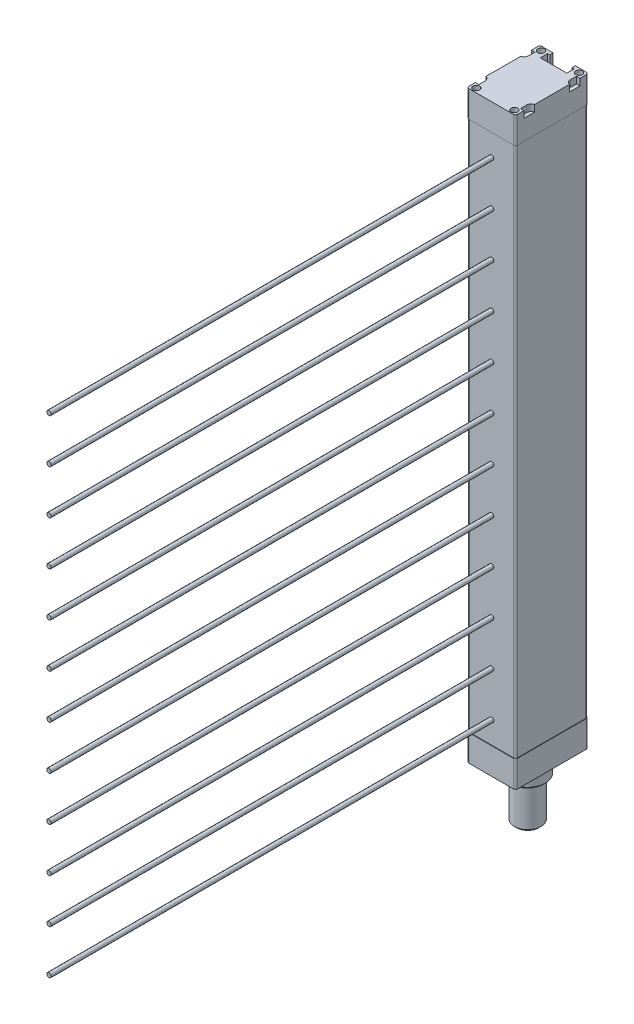
SolidWorks part; units mm, degrees
material "A6061"
ref_plane "前基準面" through (0, 0, 0) normal (0, 0, 1) x (1, 0, 0)
ref_plane "上基準面" through (0, 0, 0) normal (0, 1, 0) x (1, 0, 0)
ref_plane "右基準面" through (0, 0, 0) normal (1, 0, 0) x (0, 0, -1)
sketch "草圖1" plane through (0, 0, 0) normal (0, 1, 0) x (1, 0, 0)
  line L0 (-11, 0) -> (11, 0) construction
  line L1 (-10, 16.5) -> (-5, 16.5)
  line L2 (-11, 15.5) -> (-11, -15.5)
  line L3 (-10, -16.5) -> (10, -16.5)
  line L4 (11, 15.5) -> (11, -15.5)
  line L5 (0, 0) -> (0, 16.4415) construction
  line L6 (-5, 15) -> (-6, 15)
  line L7 (-5, 16.5) -> (-5, 15)
  line L9 (5, 16.5) -> (5, 15)
  line L10 (5, 16.5) -> (10, 16.5)
  line L11 (6, 15) -> (5, 15)
  line L12 (6, 15) -> (6, 11.7)
  line L13 (6, 11.7) -> (-6, 11.7)
  line L14 (-6, 15) -> (-6, 11.7)
  line L15 (6, 15) -> (-6, 11.7) construction
  line L16 (6, 11.7) -> (-6, 15) construction
  circle A0 centre (-8.6, 14.6) radius 1.5
  circle A1 centre (8.6, 14.6) radius 1.5
  circle A2 centre (8.6, -14.6) radius 1.5
  circle A3 centre (-8.6, -14.6) radius 1.5
  arc A4 (-10, 16.5) -> (-11, 15.5) centre (-10, 15.5) ccw
  arc A5 (11, 15.5) -> (10, 16.5) centre (10, 15.5) ccw
  arc A6 (11, -15.5) -> (10, -16.5) centre (10, -15.5) cw
  arc A7 (-11, -15.5) -> (-10, -16.5) centre (-10, -15.5) ccw
  point P21 (0, 13.35)
  dimension "D6" = 3
  dimension "D10" = 1
  dimension "D1" = 22
  dimension "D2" = 33
  dimension "D3" = 10
  dimension "D4" = 1.5
  dimension "D5" = 4.8
  dimension "D7" = 2.4
  dimension "D8" = 3.3
  dimension "D9" = 12
  dimension "D11" = 1.9
extrude "伸長1" add sketch "草圖1" along normal blind 12
sketch "草圖2" plane through (0, 12, 0) normal (0, 1, 0) x (1, 0, 0)
  line L0 (0, 0) -> (0, 14.9784) construction
  line L1 (-14.2, 12.65) -> (-9.4, 12.65)
  line L2 (-14.2, 12.65) -> (-14.2, 7.85)
  line L3 (-14.2, 7.85) -> (-11.4, 7.85)
  line L4 (-9.4, 12.65) -> (-9.4, 9.85)
  line L5 (0, 0) -> (15.7654, 0) construction
  line L6 (9.4, 12.65) -> (9.4, 9.85)
  line L7 (14.2, 7.85) -> (11.4, 7.85)
  line L8 (14.2, 12.65) -> (14.2, 7.85)
  line L9 (14.2, 12.65) -> (9.4, 12.65)
  line L10 (14.2, -12.65) -> (9.4, -12.65)
  line L11 (14.2, -12.65) -> (14.2, -7.85)
  line L12 (14.2, -7.85) -> (11.4, -7.85)
  line L13 (9.4, -12.65) -> (9.4, -9.85)
  line L14 (-9.4, -12.65) -> (-9.4, -9.85)
  line L15 (-14.2, -7.85) -> (-11.4, -7.85)
  line L16 (-14.2, -12.65) -> (-14.2, -7.85)
  line L17 (-14.2, -12.65) -> (-9.4, -12.65)
  arc A0 (-9.4, 9.85) -> (-11.4, 7.85) centre (-11.4, 9.85) cw
  arc A1 (9.4, 9.85) -> (11.4, 7.85) centre (11.4, 9.85) ccw
  arc A2 (9.4, -9.85) -> (11.4, -7.85) centre (11.4, -9.85) cw
  arc A3 (-9.4, -9.85) -> (-11.4, -7.85) centre (-11.4, -9.85) ccw
  point P17 (-15.7654, 0)
  dimension "D1" = 2
  dimension "D2" = 4.8
  dimension "D3" = 4.8
extrude "伸長2" cut sketch "草圖2" against normal blind 3
sketch "草圖3" plane through (0, 0, 0) normal (0, -1, 0) x (1, 0, 0)
  line L48 (-5.2, -16.3) -> (-5.2, -15.2)
  line L49 (-5.2, -15.2) -> (-6.2, -15.2)
  line L50 (-6.2, -15.2) -> (-6.2, -11.5)
  line L51 (-6.2, -11.5) -> (6.2, -11.5)
  line L52 (6.2, -11.5) -> (6.2, -15.2)
  line L53 (6.2, -15.2) -> (5.2, -15.2)
  line L54 (5.2, -15.2) -> (5.2, -16.3)
  line L55 (5.2, -16.3) -> (10, -16.3)
  line L56 (10.8, -15.5) -> (10.8, 15.5)
  line L57 (10, 16.3) -> (-10, 16.3)
  line L58 (-10.8, 15.5) -> (-10.8, -15.5)
  line L59 (-10, -16.3) -> (-5.2, -16.3)
  line L60 (-5.2, -16.3) -> (-5.2, -15.2)
  line L61 (-5.2, -15.2) -> (-6.2, -15.2)
  line L62 (-6.2, -15.2) -> (-6.2, -11.5)
  line L63 (-6.2, -11.5) -> (6.2, -11.5)
  line L64 (6.2, -11.5) -> (6.2, -15.2)
  line L65 (6.2, -15.2) -> (5.2, -15.2)
  line L66 (5.2, -15.2) -> (5.2, -16.3)
  line L67 (5.2, -16.3) -> (10, -16.3)
  line L68 (10.8, -15.5) -> (10.8, 15.5)
  line L69 (10, 16.3) -> (-10, 16.3)
  line L70 (-10.8, 15.5) -> (-10.8, -15.5)
  line L71 (-10, -16.3) -> (-5.2, -16.3)
  arc A12 (10, -16.3) -> (10.8, -15.5) centre (10, -15.5) ccw
  arc A13 (10.8, 15.5) -> (10, 16.3) centre (10, 15.5) ccw
  arc A14 (-10, 16.3) -> (-10.8, 15.5) centre (-10, 15.5) ccw
  arc A15 (-10.8, -15.5) -> (-10, -16.3) centre (-10, -15.5) ccw
  arc A16 (10, -16.3) -> (10.8, -15.5) centre (10, -15.5) ccw
  arc A17 (10.8, 15.5) -> (10, 16.3) centre (10, 15.5) ccw
  arc A18 (-10, 16.3) -> (-10.8, 15.5) centre (-10, 15.5) ccw
  arc A19 (-10.8, -15.5) -> (-10, -16.3) centre (-10, -15.5) ccw
  dimension "D2" = 21.6
  dimension "D3" = 32.6
  dimension "D1" = 0.2
extrude "伸長3" add sketch "草圖3" along normal blind 240
ref_plane "平面1" through (0, -120, 0) normal (0, 1, 0) x (-1, 0, 0)
mirror "鏡射1" about plane through (0, -120, 0) normal (0, 1, 0) of "伸長1"
sketch "草圖4" plane through (0, 0, 0) normal (1, 0, 0) x (0, 0, -1)
  line L0 (0, -252) -> (0, -251.8701) construction
  line L1 (-15.5, -252) -> (15.5, -252) construction
  line L2 (8, -252) -> (8, -259)
  line L3 (8, -259) -> (7, -259)
  line L4 (7, -259) -> (7, -260)
  line L5 (7, -260) -> (6, -260)
  line L6 (6, -260) -> (6, -277)
  line L7 (5, -278) -> (0, -278)
  line L8 (0, -278) -> (0, -252)
  line L9 (6, -277) -> (5, -278)
  line L10 (0, -252) -> (8, -252)
  point P12 (6, -278)
  dimension "D1" = 7
  dimension "D2" = 19
  dimension "D3" = 1
  dimension "D4" = 16
  dimension "D5" = 1
  dimension "D7" = 1
revolve "旋轉1" add sketch "草圖4" angle 360 about L0
sketch "草圖5" plane through (0, 0, 16.3) normal (0, 0, 1) x (1, 0, 0)
  line L0 (0, 12) -> (0, -278) construction
  line L1 (-10, 12) -> (10, 12) construction
  line L2 (-5, -278) -> (5, -278) construction
  line L3 (-10, 0) -> (10, 0) construction
  circle A0 centre (0, -10) radius 1
  dimension "D1" = 2
  dimension "D2" = 10
extrude "伸長4" add sketch "草圖5" along normal blind 200
pattern_linear "阵列(线性)1" count 12 spacing 20 along (0, -1, 0) of "伸長4"
